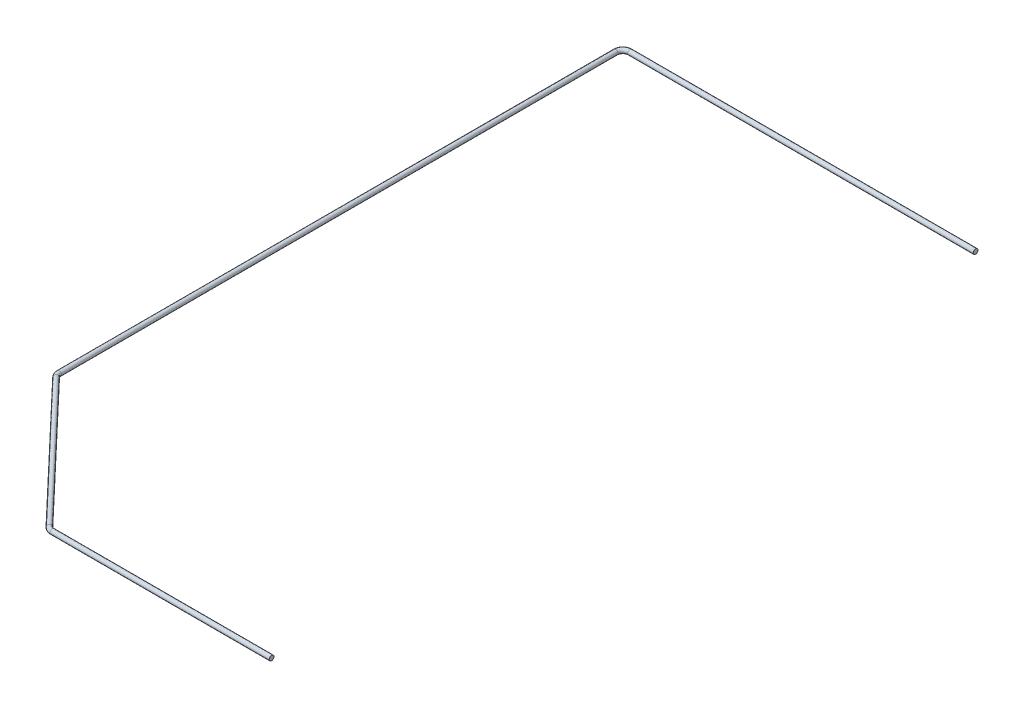
SolidWorks part; units mm, degrees
material "SWM-B"
ref_plane "Front Plane" through (0, 0, 0) normal (0, 0, 1) x (1, 0, 0)
ref_plane "Top Plane" through (0, 0, 0) normal (0, 1, 0) x (1, 0, 0)
ref_plane "Right Plane" through (0, 0, 0) normal (1, 0, 0) x (0, 0, -1)
sketch "Sketch1" plane through (0, 0, 0) normal (0, 1, 0) x (1, 0, 0)
  line L0 (0, 0) -> (-432.5, 0)
  line L1 (-441.5, -9) -> (-441.5, -705.4081)
  line L2 (-439.0269, -711.6049) -> (-280.8615, -878.1968)
  line L3 (-274.3346, -881) -> (0, -881)
  line L4 (0, 0) -> (0, -881) construction
  arc A0 (-280.8615, -878.1968) -> (-274.3346, -881) centre (-274.3346, -872) ccw
  arc A1 (-441.5, -705.4081) -> (-439.0269, -711.6049) centre (-432.5, -705.4081) ccw
  arc A2 (-432.5, 0) -> (-441.5, -9) centre (-432.5, -9) ccw
  point P9 (-278.2, -881)
  point P12 (-441.5, -709)
  point P15 (-441.5, 0)
  dimension "D5" = 9
  dimension "D1" = 441.5
  dimension "D2" = 881
  dimension "D3" = 163.3
  dimension "D4" = 709
sketch "Sketch2" plane through (0, 0, 0) normal (1, 0, 0) x (0, 0, -1)
  circle A0 centre (0, 0) radius 3
  dimension "D1" = 6
sweep "Sweep1" add profiles "Sketch2" path "Sketch1"
